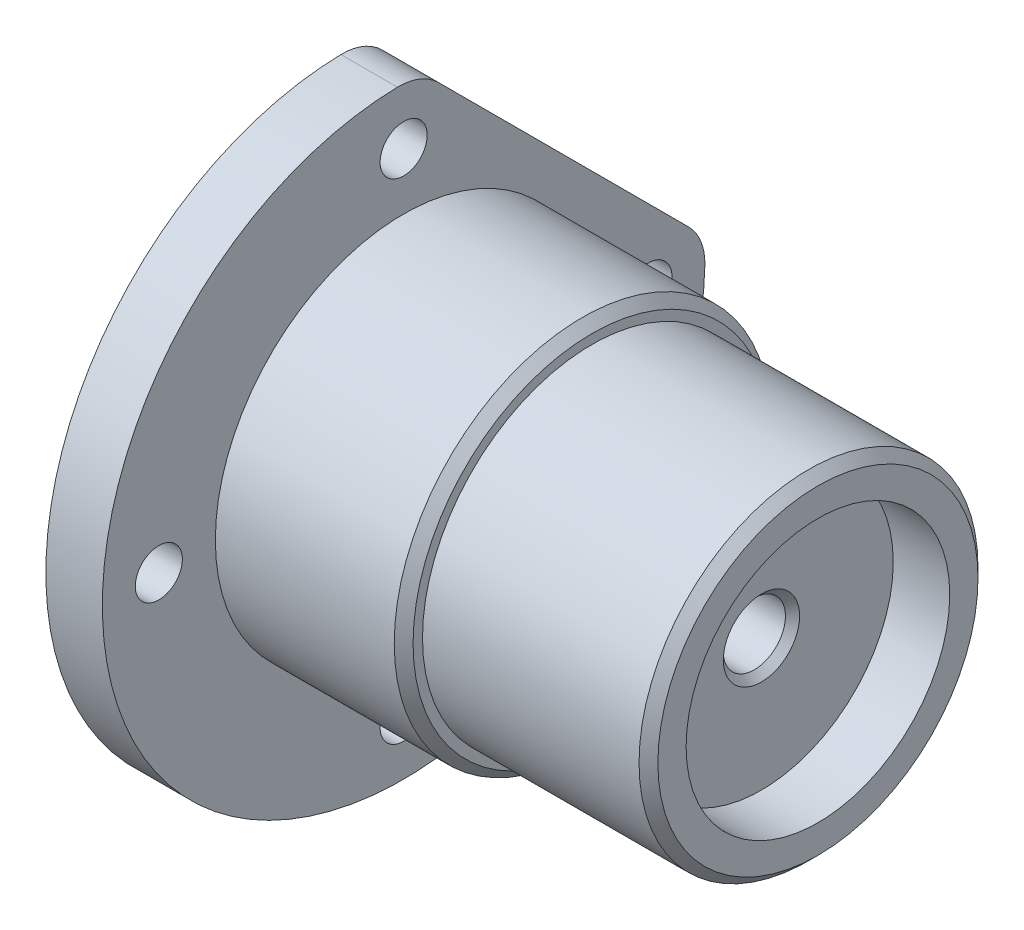
from build123d import *

# Parameters (mm, degrees)
SKETCH_2_R                   = 1.25
CUT_EXTRUDE_1_DEPTH          = 32.559467676
HOLE_WIZARD_M4_1_D           = 3.3
HOLE_WIZARD_M4_1_CSINK_D     = 4.05
HOLE_WIZARD_M4_1_CSINK_ANGLE = 90
CHAMFER_1_SIZE               = 0.5
CHAMFER_2_SIZE               = 1
CUT_EXTRUDE_2_DEPTH          = 10
FILLET_1_R                   = 3
HOLE_WIZARD_M3_1_D           = 2.5


with BuildPart() as part:
    # 草图1 → 旋转1 (revolve)
    with BuildSketch(Plane(origin=(0, 0, 0), x_dir=(1, 0, 0), z_dir=(0, 1, 0)), mode=Mode.PRIVATE) as revolve_1_sk:
        Polygon((0, 7), (0, 16), (3, 16), (3, 10), (13, 10), (13, 9), (25, 9), (25, 7), (22, 7), (22, 0), (19, 0), (19, 7), align=None)
    revolve(revolve_1_sk.sketch.rotate(Axis((-407.867518885, 0, 0), (1, 0, 0)), 180), axis=Axis((-407.867518885, 0, 0), (1, 0, 0)))

    # 草图2 → 切除-拉伸1 (cut, through all)
    with BuildSketch(Plane(origin=(3, 0, 0), x_dir=(0, 0, -1), z_dir=(1, 0, 0))):
        with Locations((0, 13)):
            Circle(SKETCH_2_R)
        with Locations((13, 0)):
            Circle(SKETCH_2_R)
        with Locations((0, -13)):
            Circle(SKETCH_2_R)
        with Locations((-13, 0)):
            Circle(SKETCH_2_R)
    extrude(amount=-CUT_EXTRUDE_1_DEPTH, mode=Mode.SUBTRACT)

    # M4 螺纹孔1 (through all)
    with Locations(Plane(origin=(22, 0, 0), x_dir=(0, 0, -1), z_dir=(1, 0, 0))):
        with Locations((0, 0)):
            CounterSinkHole(HOLE_WIZARD_M4_1_D / 2, HOLE_WIZARD_M4_1_CSINK_D / 2, counter_sink_angle=HOLE_WIZARD_M4_1_CSINK_ANGLE)

    # 倒角1
    chamfer_1_edges = [part.edges().sort_by_distance(p)[0] for p in [
        (25, 0, -9),
        (13, 0, -10),
    ]]
    chamfer(chamfer_1_edges, length=CHAMFER_1_SIZE)

    # 倒角2
    chamfer_2_edges = [part.edges().sort_by_distance(p)[0] for p in [
        (0, 0, -7),
    ]]
    chamfer(chamfer_2_edges, length=CHAMFER_2_SIZE)

    # 草图5 → 切除-拉伸2 (cut)
    with BuildSketch(Plane(origin=(3, 0, 0), x_dir=(0, 0, -1), z_dir=(1, 0, 0))):
        with BuildLine():
            Line((1.001966601, 15.968596148), (15.968596148, 1.001966601))
            ThreePointArc((15.968596148, 1.001966601), (11.313708499, 11.313708499), (1.001966601, 15.968596148))
        make_face()
    extrude(amount=-CUT_EXTRUDE_2_DEPTH, mode=Mode.SUBTRACT)

    # 圆角1
    fillet_1_edges = [part.edges().sort_by_distance(p)[0] for p in [
        (1.5, 15.968596148, -1.001966601),
        (1.5, 1.001966601, -15.968596148),
    ]]
    fillet(fillet_1_edges, radius=FILLET_1_R)

    # M3 螺纹孔1 (through all)
    with Locations(Plane(origin=(3, 13, 0), x_dir=(0, 0, 1), z_dir=(1, 0, 0))):
        with Locations((0, 0), (13, 13), (0, 26), (-13, 13)):
            Hole(HOLE_WIZARD_M3_1_D / 2)


solid = part.part
